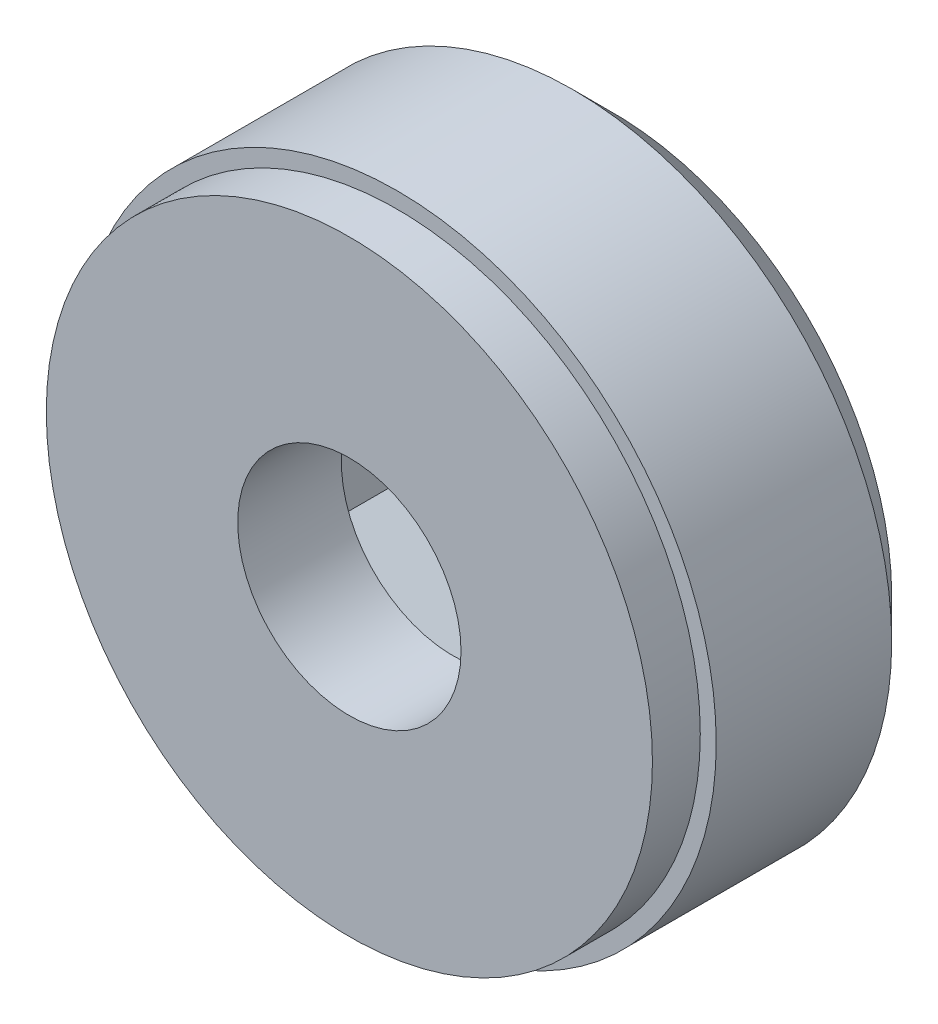
from build123d import *

# Parameters (mm, degrees)
SKETCH1_R           = 40
BOSS_EXTRUDE1_DEPTH = 33
CUT_EXTRUDE1_START  = -6
SKETCH2_R           = 40
SKETCH2_R_2         = 38
CUT_EXTRUDE1_DEPTH  = 6
CHAMFER1_SIZE       = 5
SKETCH3_R           = 14
CUT_EXTRUDE2_DEPTH  = 13
CUT_EXTRUDE3_DEPTH  = 20


with BuildPart() as part:
    # Sketch1 → Boss-Extrude1 (new body)
    with BuildSketch(Plane.XY):
        Circle(SKETCH1_R)
    extrude(amount=BOSS_EXTRUDE1_DEPTH)

    # Sketch2 → Cut-Extrude1 (cut)
    with BuildSketch(Plane.XY.offset(33).offset(CUT_EXTRUDE1_START)):
        Circle(SKETCH2_R)
        Circle(SKETCH2_R_2, mode=Mode.SUBTRACT)
    extrude(amount=CUT_EXTRUDE1_DEPTH, mode=Mode.SUBTRACT)

    # Chamfer1
    chamfer1_edges = [part.edges().sort_by_distance(p)[0] for p in [
        (-40, 0, 0),
    ]]
    chamfer(chamfer1_edges, length=CHAMFER1_SIZE)

    # Sketch3 → Cut-Extrude2 (cut)
    with BuildSketch(Plane.XY.offset(33)):
        Circle(SKETCH3_R)
    extrude(amount=-CUT_EXTRUDE2_DEPTH, mode=Mode.SUBTRACT)

    # Sketch4 → Cut-Extrude3 (cut)
    with BuildSketch(Plane(origin=(0, 0, 0), x_dir=(-1, 0, 0), z_dir=(0, 0, -1))):
        Polygon((-19.5, -11.258330249), (0, -22.516660498), (19.5, -11.258330249), (19.5, 11.258330249), (0, 22.516660498), (-19.5, 11.258330249), align=None)
    extrude(amount=-CUT_EXTRUDE3_DEPTH, mode=Mode.SUBTRACT)


solid = part.part
